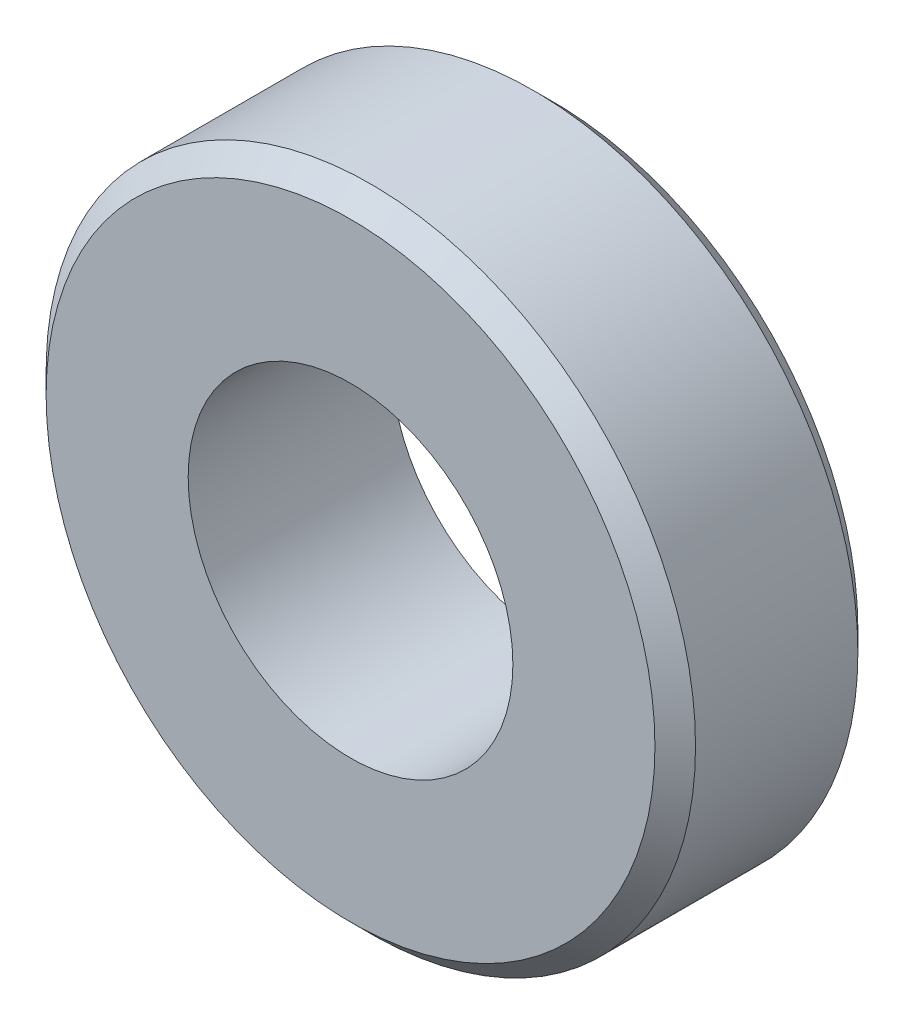
SolidWorks part; units mm, degrees
material "普通碳钢"
ref_plane "前视基准面" through (0, 0, 0) normal (0, 0, 1) x (1, 0, 0)
ref_plane "上视基准面" through (0, 0, 0) normal (0, 1, 0) x (1, 0, 0)
ref_plane "右视基准面" through (0, 0, 0) normal (1, 0, 0) x (0, 0, -1)
sketch "草图1" plane through (0, 0, 0) normal (0, 0, 1) x (1, 0, 0)
  circle A0 centre (0, 0) radius 4
  circle A1 centre (0, 0) radius 8
  dimension "D1" = 16
  dimension "D2" = 8
extrude "凸台-拉伸1" add sketch "草图1" along normal mid plane 5
chamfer "倒角1" distance 0.5 angle 45 2 edges at (8, 0, -2.5) (8, 0, 2.5)
